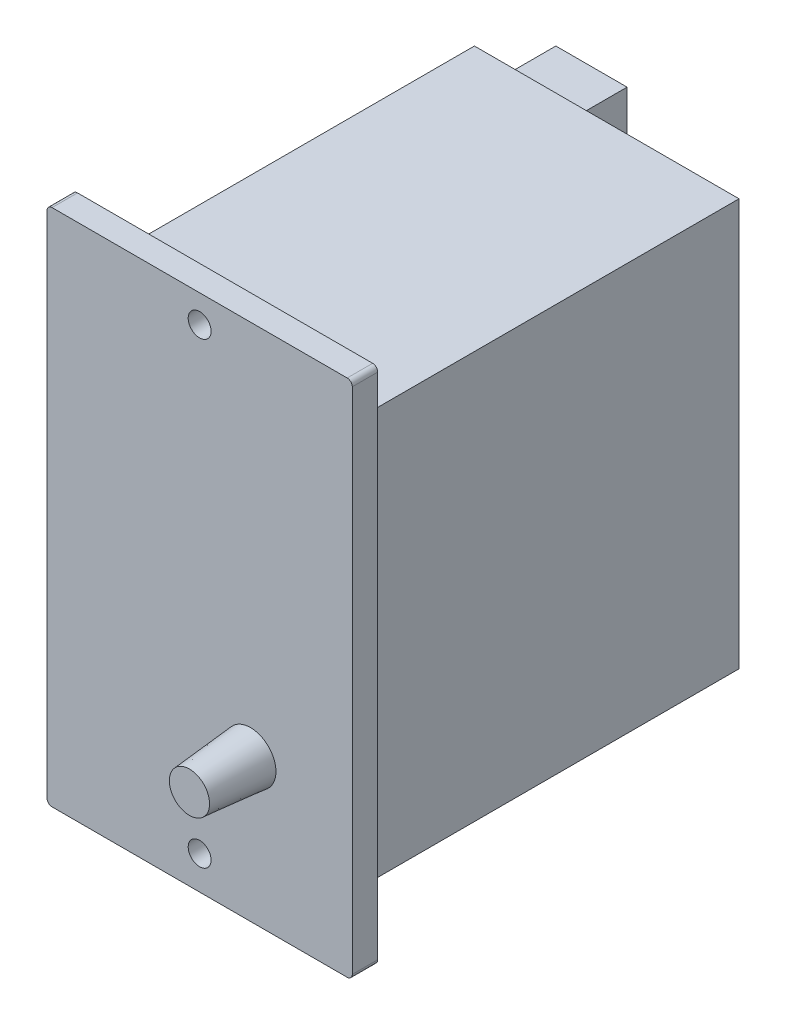
from build123d import *

# Parameters (mm, degrees)
SKETCH_1_W      = 60
SKETCH_1_H      = 102
SKETCH_1_R      = 2.25
EXTRUDE_1_DEPTH = 5
SKETCH_2_W      = 52
SKETCH_2_H      = 80
EXTRUDE_2_DEPTH = 75
SKETCH_3_R      = 5
EXTRUDE_3_DEPTH = 12
EXTRUDE_3_TAPER = 5
FILLET_1_R      = 1
SKETCH_4_W      = 14
SKETCH_4_H      = 72
EXTRUDE_4_DEPTH = 12


with BuildPart() as part:
    # 草图1 → 凸台-拉伸1 (new body)
    with BuildSketch(Plane.XY):
        Rectangle(SKETCH_1_W, SKETCH_1_H)
        with Locations((0, 45.563491435)):
            Circle(SKETCH_1_R, mode=Mode.SUBTRACT)
        with Locations((0, -44.436508565)):
            Circle(SKETCH_1_R, mode=Mode.SUBTRACT)
    extrude(amount=EXTRUDE_1_DEPTH)

    # 草图2 → 凸台-拉伸2 (add)
    with BuildSketch(Plane(origin=(0, 0, 0), x_dir=(-1, 0, 0), z_dir=(0, 0, -1))):
        Rectangle(SKETCH_2_W, SKETCH_2_H)
    extrude(amount=EXTRUDE_2_DEPTH)

    # 草图3 → 凸台-拉伸3 (add)
    with BuildSketch(Plane.XY.offset(5)):
        with Locations((10, -23)):
            Circle(SKETCH_3_R)
    extrude(amount=EXTRUDE_3_DEPTH, taper=EXTRUDE_3_TAPER)

    # 圆角1
    fillet_1_edges = [part.edges().sort_by_distance(p)[0] for p in [
        (30, -51, 2.5),
        (-30, -51, 2.5),
        (-30, 51, 2.5),
        (30, 51, 2.5),
    ]]
    fillet(fillet_1_edges, radius=FILLET_1_R)

    # 草图4 → 凸台-拉伸4 (add)
    with BuildSketch(Plane(origin=(0, 0, -75), x_dir=(-1, 0, 0), z_dir=(0, 0, -1))):
        with Locations((15, 0)):
            Rectangle(SKETCH_4_W, SKETCH_4_H)
    extrude(amount=EXTRUDE_4_DEPTH)


solid = part.part
